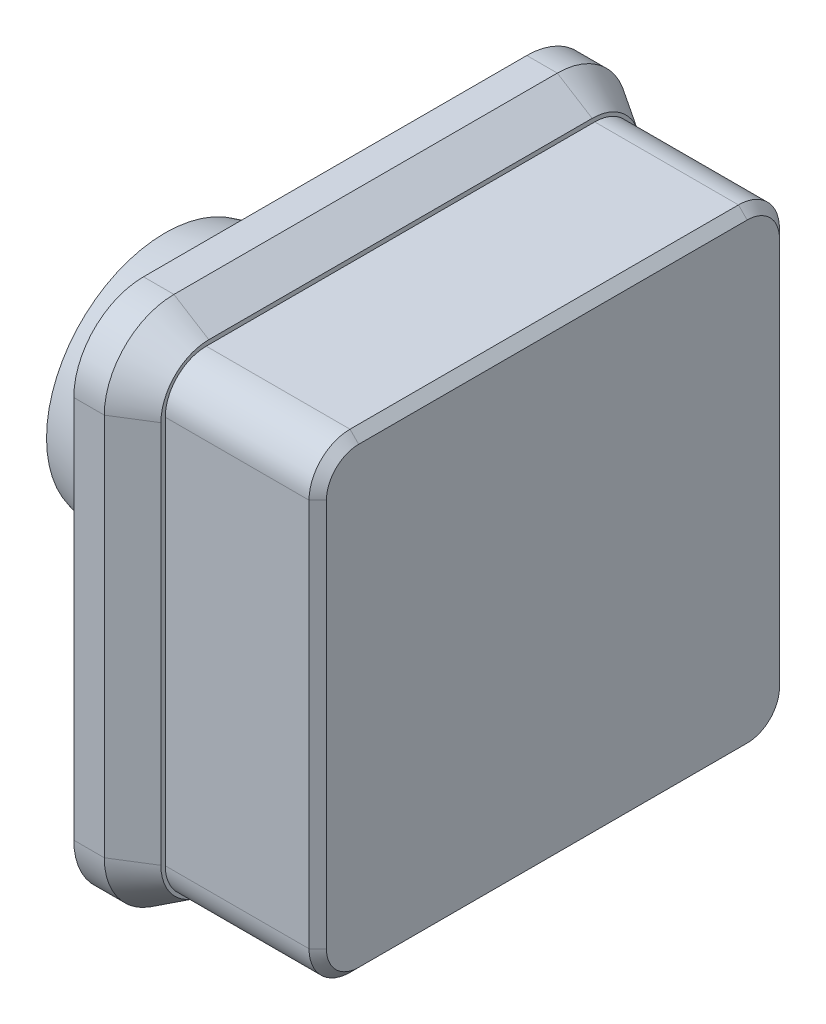
SolidWorks part; units mm, degrees
material "Q235B"
ref_plane "Front Plane" through (0, 0, 0) normal (0, 0, 1) x (1, 0, 0)
ref_plane "Top Plane" through (0, 0, 0) normal (0, 1, 0) x (1, 0, 0)
ref_plane "Right Plane" through (0, 0, 0) normal (1, 0, 0) x (0, 0, -1)
other "Configuration Table"
sketch "Sketch1" plane through (0, 0, 0) normal (0, 1, 0) x (1, 0, 0)
  line L0 (30, 35) -> (0, 26.9615)
  line L1 (0, 0) -> (30, 0)
  line L2 (0, 0) -> (0, 26.9615)
  line L4 (30, 0) -> (30, 35)
  line L5 (30, 0) -> (40, 0)
  line L6 (30, 0) -> (30, 35)
  line L7 (30, 35) -> (40, 35)
  line L8 (40, 0) -> (40, 35)
  dimension "D1" = 35
  dimension "D2" = 10
  dimension "D3" = 15
  dimension "D4" = 30
revolve "Revolve1" add sketch "Sketch1" angle 360 about L1
sketch "Sketch2" plane through (40, 0, 0) normal (1, 0, 0) x (0, 0, -1)
  line L1 (-44, -60) -> (44, -60)
  line L2 (-60, -44) -> (-60, 44)
  line L3 (-44, 60) -> (44, 60)
  line L4 (60, -44) -> (60, 44)
  line L5 (-60, -60) -> (60, 60) construction
  line L6 (-60, 60) -> (60, -60) construction
  arc A0 (-44, -60) -> (-60, -44) centre (-44, -44) cw
  arc A1 (44, -60) -> (60, -44) centre (44, -44) ccw
  arc A2 (44, 60) -> (60, 44) centre (44, 44) cw
  arc A3 (-44, 60) -> (-60, 44) centre (-44, 44) ccw
  point P0 (0, 0)
  dimension "D3" = 16
  dimension "D1" = 120
  dimension "D2" = 120
extrude "Boss-Extrude1" add sketch "Sketch2" along normal blind 15
chamfer "Chamfer1" distance 8 distance2 5 8 edges at (55, 0, 60) (55, 55.3137, 55.3137) (55, 60, 0) (55, 55.3137, -55.3137) (55, 0, -60) (55, -55.3137, -55.3137) (55, -60, 0) (55, -55.3137, 55.3137)
sketch "Sketch3" plane through (55, 0, 0) normal (1, 0, 0) x (0, 0, -1)
  line L1 (-44.5911, -54) -> (44.5911, -54)
  line L2 (-54, -44.5911) -> (-54, 44.5911)
  line L3 (-44.5911, 54) -> (44.5911, 54)
  line L4 (54, -44.5911) -> (54, 44.5911)
  line L5 (-54, -54) -> (54, 54) construction
  line L6 (-54, 54) -> (54, -54) construction
  arc A1 (44.5911, 54) -> (54, 44.5911) centre (44.5911, 44.5911) cw
  arc A2 (54, -44.5911) -> (44.5911, -54) centre (44.5911, -44.5911) cw
  arc A3 (-44.5911, -54) -> (-54, -44.5911) centre (-44.5911, -44.5911) cw
  arc A4 (-54, 44.5911) -> (-44.5911, 54) centre (-44.5911, 44.5911) cw
  point P0 (0, 0)
  dimension "D1" = 108
  dimension "D3" = 9.4089
  dimension "D2" = 108
extrude "Boss-Extrude2" add sketch "Sketch3" along normal blind 35
chamfer "Chamfer2" distance 2 angle 45 8 edges at (90, -54, 0) (90, 0, 54) (90, 54, 0) (90, 0, -54) (90, -51.2442, -51.2442) (90, -51.2442, 51.2442) (90, 51.2442, 51.2442) (90, 51.2442, -51.2442)
chamfer "Chamfer3" distance 1 angle 45 1 edges at (0, 0, 26.9615)
